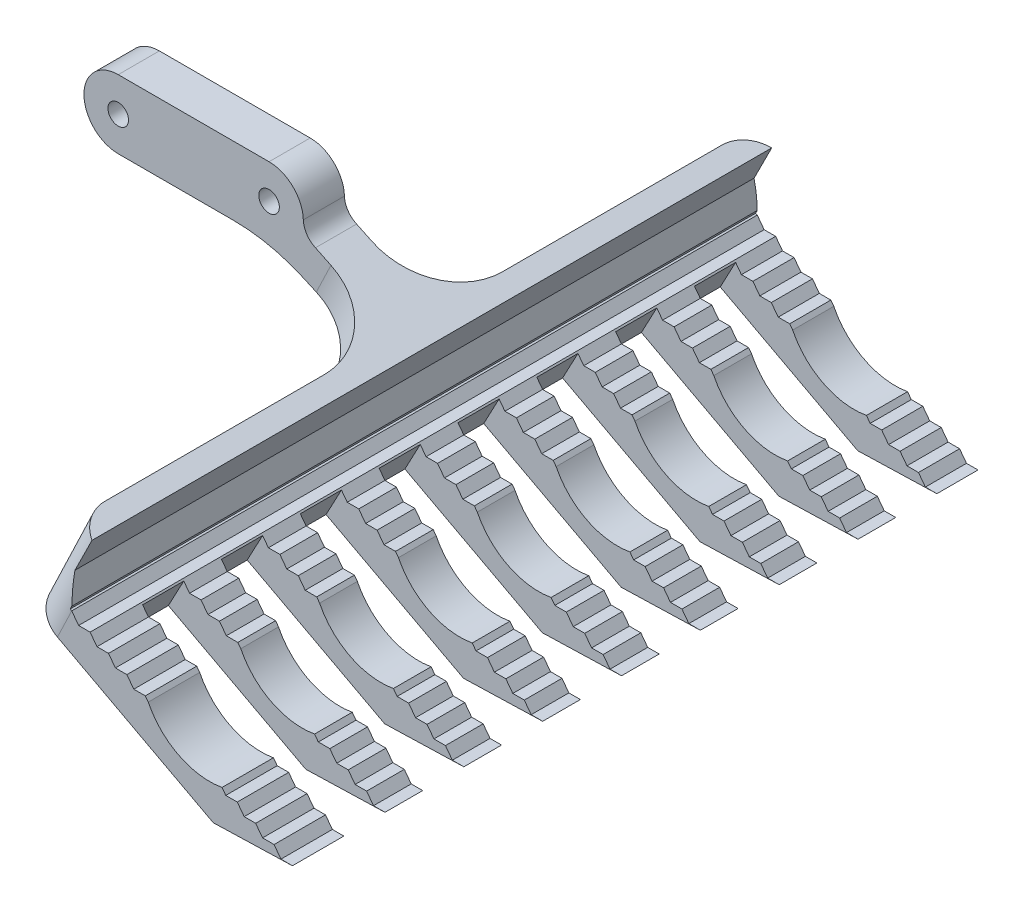
from build123d import *

# Parameters (mm, degrees)
SKETCH1_R               = 1.499999999999788
SKETCH1_R_2             = 1.5000000000000013
BOSS_EXTRUDE1_DEPTH     = 6.000000000000001
CUT_EXTRUDE1_DEPTH      = 10
BOSS_EXTRUDE2_START     = -3
BOSS_EXTRUDE2_DEPTH     = 50
FILLET1_R               = 10
FILLET2_R               = 5
CUT_EXTRUDE2_DEPTH      = 100
SKETCH10_R              = 10.000000000000002
CUT_EXTRUDE4_DEPTH      = 129.13418296706914
CUT_EXTRUDE5_DEPTH      = 97.13435681961771
CUT_EXTRUDE5_DEPTH_BACK = 97.13435681961771
SKETCH13_W              = 45
SKETCH13_H              = 6.0000000000000036
SKETCH13_H_2            = 6
SKETCH13_H_3            = 5.999999999999998
SKETCH13_H_4            = 5.999999999999999
SKETCH13_H_5            = 5.9999999999999964
CUT_EXTRUDE6_DEPTH      = 97.05919448256036
CUT_EXTRUDE6_DEPTH_BACK = 97.05919448256036
CUT_EXTRUDE7_DEPTH      = 129.13418296706914


with BuildPart() as part:
    # Sketch1 → Boss-Extrude1 (new body)
    with BuildSketch(Plane.XY.offset(6)):
        with BuildLine():
            Line((35.197003070326204, -5.91650592956903), (35.197003070326204, -5.3685569000436395))
            Line((35.197003070326204, -5.3685569000436395), (34.945301708965154, -5.255713659117091))
            Line((34.945301708965154, -5.255713659117091), (29.01160192717406, -7.52704716735931))
            Line((29.01160192717406, -7.52704716735931), (17.76879404095149, -2.4866498006710818))
            ThreePointArc((17.76879404095149, -2.4866498006710818), (16.503827212867638, -1.4191215987882164), (15.9975417301403, 0.1567694342301625))
            ThreePointArc((15.9975417301403, 0.1567694342301625), (14.479666135483196, 3.590532493319067), (11.000000000000211, 5.000000000000988))
            Line((11.000000000000211, 5.000000000000988), (-10.999999999999787, 5.000000000000985))
            ThreePointArc((-10.999999999999787, 5.000000000000985), (-15.999999999999787, 9.8604e-13), (-10.999999999999787, -4.999999999999015))
            Line((-10.999999999999787, -4.999999999999015), (5.805088555171512, -4.999999999999016))
            ThreePointArc((5.805088555171512, -4.999999999999016), (11.034404003531415, -5.553031681993929), (16.03236128244425, -7.18765920467546))
            Line((16.03236128244425, -7.18765920467546), (30.60269125669545, -13.719857706793727))
            ThreePointArc((30.60269125669545, -13.719857706793727), (37.870669942651325, -13.928931417022774), (43.157744395280794, -8.937531840934865))
            Line((43.157744395280794, -8.937531840934865), (42.90604303392061, -8.824688600008706))
            Line((42.90604303392061, -8.824688600008706), (42.4969521248297, -9.1892332022963))
            Line((42.4969521248297, -9.1892332022963), (42.49695212482971, -8.641284172770877))
            Line((42.49695212482971, -8.641284172770877), (41.99354940210771, -8.41559769091782))
            Line((41.99354940210771, -8.41559769091782), (41.58445849301675, -8.78014229320539))
            Line((41.58445849301675, -8.78014229320539), (41.58445849301681, -8.232193263679989))
            Line((41.58445849301681, -8.232193263679989), (41.08105577029475, -8.006506781826907))
            Line((41.08105577029475, -8.006506781826907), (40.67196486120385, -8.371051384114478))
            Line((40.67196486120385, -8.371051384114478), (40.671964861203854, -7.823102354589077))
            Line((40.671964861203854, -7.823102354589077), (40.16856213848181, -7.597415872736))
            Line((40.16856213848181, -7.597415872736), (39.7594712293909, -7.961960475023569))
            Line((39.7594712293909, -7.961960475023569), (39.759471229390904, -7.414011445498166))
            Line((39.759471229390904, -7.414011445498166), (39.25606850666886, -7.18832496364509))
            Line((39.25606850666886, -7.18832496364509), (38.84697759757795, -7.552869565932659))
            Line((38.84697759757795, -7.552869565932659), (38.84697759757796, -7.00492053640726))
            Line((38.84697759757796, -7.00492053640726), (38.34357487485592, -6.779234054554182))
            Line((38.34357487485592, -6.779234054554182), (37.934483965765004, -7.14377865684176))
            Line((37.934483965765004, -7.14377865684176), (37.934483965765004, -6.595829627316349))
            Line((37.934483965765004, -6.595829627316349), (37.43108124304296, -6.370143145463272))
            Line((37.43108124304296, -6.370143145463272), (37.021990333952054, -6.73468774775084))
            Line((37.021990333952054, -6.73468774775084), (37.0219903339521, -6.186738718225458))
            Line((37.0219903339521, -6.186738718225458), (36.51858761123001, -5.961052236372362))
            Line((36.51858761123001, -5.961052236372362), (36.109496702139104, -6.325596838659941))
            Line((36.109496702139104, -6.325596838659941), (36.10949670213915, -5.777647809134549))
            Line((36.10949670213915, -5.777647809134549), (35.6060939794171, -5.55196132728147))
            Line((35.6060939794171, -5.55196132728147), (35.197003070326204, -5.91650592956903))
        make_face()
        with Locations((-10.999999999999787, 9.8543e-13)):
            Circle(SKETCH1_R, mode=Mode.SUBTRACT)
        with Locations((11.000000000000211, 9.7482e-13)):
            Circle(SKETCH1_R, mode=Mode.SUBTRACT)
        with Locations((36.54982169076239, -11.45454545454544)):
            Circle(SKETCH1_R_2, mode=Mode.SUBTRACT)
    extrude(amount=-BOSS_EXTRUDE1_DEPTH)

    # Sketch6 → Cut-Extrude1 (cut)
    with BuildSketch(Plane.XY.offset(6)):
        Polygon((17.7687940409514, -2.4866498006718), (29.049191934368057, -7.873012737172492), (25.37664072795702, -15.564258087820532), (48.33969324068796, -22.932767788258534), (43.962048995801126, 0.8987256866975355), align=None)
    extrude(amount=-CUT_EXTRUDE1_DEPTH, mode=Mode.SUBTRACT)

    # Sketch7 → Boss-Extrude2 (add, symmetric)
    with BuildSketch(Plane.XY.offset(6).offset(BOSS_EXTRUDE2_START)):
        Polygon((29.049191934368057, -7.873012737172492), (27.023536599966086, -12.115244171696116), (24.740243361962573, -16.89703413566024), (22.714588027560602, -21.139265570183863), (58.032491741917646, -39.91812808161954), (69.46158575139046, -39.257748231761035), (28.979950972821662, -19.016892008260545), (33.49134140531283, -9.994128454434303), align=None)
    extrude(amount=BOSS_EXTRUDE2_DEPTH, both=True)

    # Fillet1
    fillet1_edges = [part.edges().sort_by_distance(p)[0] for p in [
        (28.036364267167276, -9.994128454433872, -8.9e-16),
        (28.03636426716728, -9.994128454433874, 6),
    ]]
    fillet(fillet1_edges, radius=FILLET1_R)

    # Fillet2
    fillet2_edges = [part.edges().sort_by_distance(p)[0] for p in [
        (25.88188998096433, -14.506139153678177, -47),
        (25.88188998096433, -14.506139153678177, 53),
    ]]
    fillet(fillet2_edges, radius=FILLET2_R)

    # Sketch8 → Cut-Extrude2 (cut)
    with BuildSketch(Plane.XY.offset(53.00000000000001)):
        Polygon((34.5282929549287, -11.451095925705737), (33.522064038209415, -10.10945307993969), (33.522064038209415, -5.212737210445795), (72.12356025434019, -25.323771299742504), (71.08799164532884, -28.89245292066436), (69.41094001868245, -28.892452920664358), (68.40471110196317, -27.550810074898312), (66.72765947531678, -27.55081007489831), (65.72143055859749, -26.209167229132266), (64.0443789319511, -26.20916722913226), (63.038150015231814, -24.867524383366217), (61.36109838858543, -24.867524383366217), (60.354869471866145, -23.52588153760017), (58.67781784521976, -23.525881537600164), (57.67158892850047, -22.18423869183412), (55.99453730185408, -22.18423869183412), (54.9883083851348, -20.842595846068075), (53.31125675848841, -20.84259584606807), (52.305027841769125, -19.500953000302022), (50.627976215122736, -19.500953000302022), (49.62174729840345, -18.15931015453598), (47.94469567175706, -18.159310154535977), (46.93846675503778, -16.81766730876993), (45.26141512839139, -16.817667308769927), (44.255186211672104, -15.476024463003883), (42.57813458502572, -15.47602446300388), (41.57190566830643, -14.134381617237835), (39.89485404166005, -14.134381617237832), (38.88862512494076, -12.792738771471788), (37.21157349829438, -12.792738771471784), (36.20534458157509, -11.451095925705738), align=None)
        Polygon((43.635747099351576, -27.183331553023724), (45.312798725997965, -27.183331553023727), (46.31902764271725, -28.52497439878977), (47.99607926936364, -28.52497439878977), (49.00230818608293, -29.866617244555815), (50.67935981272932, -29.866617244555822), (51.6855887294486, -31.208260090321865), (53.362640356094985, -31.208260090321865), (54.36886927281427, -32.54990293608791), (56.04592089946066, -32.54990293608792), (57.05214981617995, -33.891545781853964), (58.72920144282633, -33.891545781853964), (59.73543035954562, -35.23318862762001), (61.412481986192, -35.23318862762001), (62.41871090291129, -36.574831473386055), (64.09576252955767, -36.574831473386055), (65.10199144627695, -37.9164743191521), (66.77904307292334, -37.91647431915211), (67.81461168193471, -34.34779269823025), (29.213115465803927, -14.236758608933542), (29.213115465803927, -19.133474478427438), (30.219344382523218, -20.475117324193484), (31.896396009169603, -20.475117324193487), (32.902624925888894, -21.81676016995953), (34.579676552535275, -21.816760169959533), (35.58590546925456, -23.15840301572558), (37.262957095900944, -23.158403015725582), (38.26918601262023, -24.500045861491625), (39.94623763926662, -24.50004586149163), (40.95246655598591, -25.841688707257674), (42.629518182632296, -25.841688707257678), align=None)
    extrude(amount=-CUT_EXTRUDE2_DEPTH, mode=Mode.SUBTRACT)

    # Sketch10 → Cut-Extrude4 (cut, through all)
    with BuildSketch(Plane(origin=(0, 0, -47), x_dir=(-1, 0, 0), z_dir=(0, 0, -1))):
        with Locations((-49.339905408093855, -20.64068761944537)):
            Circle(SKETCH10_R)
    extrude(amount=-CUT_EXTRUDE4_DEPTH, mode=Mode.SUBTRACT)

    # Sketch13 → Cut-Extrude5 (cut, two sides: drawn at the far end of the back side and taken through both)
    with BuildSketch(Plane(origin=(0.93408704378427, 1.7567622241821879, 0), x_dir=(-0.8829475928589262, 0.4694715627858923, 0), z_dir=(-0.4694715627858923, -0.8829475928589262, 0)).offset(-CUT_EXTRUDE5_DEPTH_BACK)):
        with Locations((-60.52013180591146, 26.5)):
            Rectangle(SKETCH13_W, SKETCH13_H)
        with Locations((-60.52013180591146, 38)):
            Rectangle(SKETCH13_W, SKETCH13_H_2)
        with Locations((-60.52013180591146, 15.000000000000004)):
            Rectangle(SKETCH13_W, SKETCH13_H_2)
        with Locations((-60.52013180591146, 3.5)):
            Rectangle(SKETCH13_W, SKETCH13_H_3)
        with Locations((-60.52013180591146, -7.9999999999999964)):
            Rectangle(SKETCH13_W, SKETCH13_H_4)
        with Locations((-60.52013180591146, -19.499999999999993)):
            Rectangle(SKETCH13_W, SKETCH13_H_2)
        with Locations((-60.52013180591146, -31)):
            Rectangle(SKETCH13_W, SKETCH13_H_5)
        with Locations((-60.52013180591146, -42.5)):
            Rectangle(SKETCH13_W, SKETCH13_H_2)
    extrude(amount=CUT_EXTRUDE5_DEPTH + CUT_EXTRUDE5_DEPTH_BACK, mode=Mode.SUBTRACT)

    # Sketch11 → Cut-Extrude6 (cut, two sides: drawn at the far end of the back side and taken through both)
    with BuildSketch(Plane.XY.offset(-CUT_EXTRUDE6_DEPTH_BACK)):
        Polygon((29.213115465803927, -14.236758608933542), (31.75014416377548, -9.16271094810436), (33.49134140531283, -9.994128454434303), (30.92427262051907, -15.12825617363776), align=None)
    extrude(amount=CUT_EXTRUDE6_DEPTH + CUT_EXTRUDE6_DEPTH_BACK, mode=Mode.SUBTRACT)

    # Sketch15 → Cut-Extrude7 (cut, through all)
    with BuildSketch(Plane.XY.offset(53.00000000000001)):
        Polygon((49.86054410299138, -35.573026446958686), (61.412481986192, -35.23318862762001), (69.46158575139046, -39.257748231761035), (58.03249174191769, -39.91812808161955), align=None)
    extrude(amount=-CUT_EXTRUDE7_DEPTH, mode=Mode.SUBTRACT)


solid = part.part
